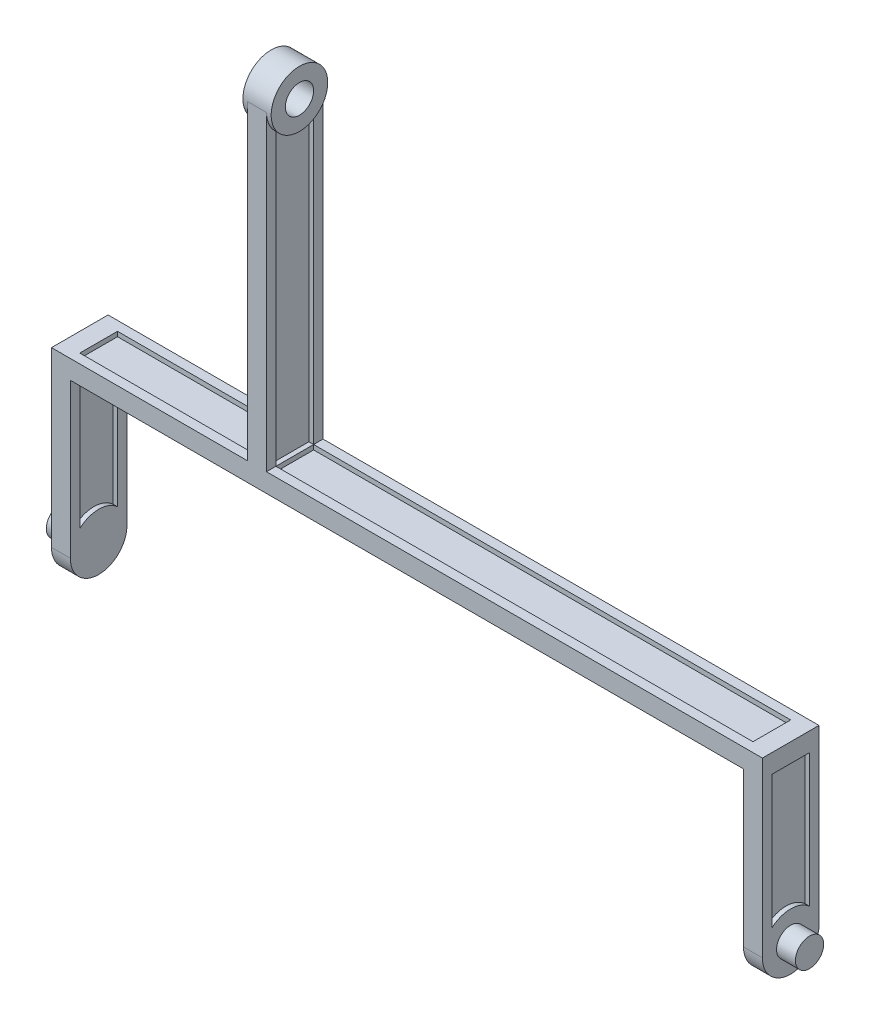
from build123d import *

# Parameters (mm, degrees)
SKETCH_2_R           = 30
SKETCH_2_R_2         = 15
EXTRUDE_1_DEPTH      = 15
EXTRUDE_2_DEPTH      = 10
CUT_EXTRUDE_1_DEPTH  = 5
CUT_EXTRUDE_START    = -5
CUT_EXTRUDE_2_DEPTH  = 5
EXTRUDE_3_DEPTH      = 536
EXTRUDE_3_DEPTH_BACK = 218
SKETCH_6_W           = 60
SKETCH_6_H           = 20
SKETCH_8_W           = 188
SKETCH_8_H           = 40
SKETCH_8_W_2         = 506
CUT_EXTRUDE_3_DEPTH  = 5
SKETCH_9_W           = 714
SKETCH_9_H           = 40
CUT_EXTRUDE_4_DEPTH  = 5
EXTRUDE_4_DEPTH      = 20
EXTRUDE_START        = -20
EXTRUDE_5_DEPTH      = 20
CUT_EXTRUDE_5_DEPTH  = 5
CUT_EXTRUDE_6_DEPTH  = 5
CUT_EXTRUDE_7_DEPTH  = 5
CUT_EXTRUDE_8_DEPTH  = 5
SKETCH_17_R          = 15
EXTRUDE_6_DEPTH      = 20
SKETCH_18_R          = 15.5
EXTRUDE_7_DEPTH      = 20


with BuildPart() as part:
    # 草图2 → 凸台-拉伸1 (new, symmetric)
    with BuildSketch(Plane(origin=(0, 0, 0), x_dir=(0, 0, -1), z_dir=(1, 0, 0))):
        with Locations((0, 34.284448819)):
            Circle(SKETCH_2_R)
        with Locations((0, 34.284448819)):
            Circle(SKETCH_2_R_2, mode=Mode.SUBTRACT)
    extrude(amount=EXTRUDE_1_DEPTH, both=True)

    # 草图3 → 凸台-拉伸2 (add, symmetric)
    with BuildSketch(Plane(origin=(0, 0, 0), x_dir=(0, 0, -1), z_dir=(1, 0, 0))):
        with BuildLine():
            Line((-30, 34.284448819), (-30, -315.715551181))
            Line((-30, -315.715551181), (30, -315.715551181))
            Line((30, -315.715551181), (30, 34.284448819))
            ThreePointArc((30, 34.284448819), (0, 4.284448819), (-30, 34.284448819))
        make_face()
    extrude(amount=EXTRUDE_2_DEPTH, both=True)

    # 草图4 → 切除-拉伸1 (cut)
    with BuildSketch(Plane(origin=(10, 0, 0), x_dir=(0, 0, -1), z_dir=(1, 0, 0))):
        with BuildLine():
            Line((-20, -315.715551181), (-20, 11.923769044))
            ThreePointArc((-20, 11.923769044), (0, 4.284448819), (20, 11.923769044))
            Line((20, 11.923769044), (20, -315.715551181))
            Line((20, -315.715551181), (-20, -315.715551181))
        make_face()
    extrude(amount=-CUT_EXTRUDE_1_DEPTH, mode=Mode.SUBTRACT)

    # 草图5 → 切除-拉伸2 (cut)
    with BuildSketch(Plane.ZY.offset(10).offset(CUT_EXTRUDE_START)):
        with BuildLine():
            Line((-20, 11.923769044), (-20, -315.715551181))
            Line((-20, -315.715551181), (20, -315.715551181))
            Line((20, -315.715551181), (20, 11.923769044))
            ThreePointArc((20, 11.923769044), (0, 4.284448819), (-20, 11.923769044))
        make_face()
    extrude(amount=CUT_EXTRUDE_2_DEPTH, mode=Mode.SUBTRACT)

    # 草图6 → 凸台-拉伸3 (add, two sides: drawn at the far end of the back side and taken through both)
    with BuildSketch(Plane(origin=(0, 0, 0), x_dir=(0, 0, -1), z_dir=(1, 0, 0)).offset(-EXTRUDE_3_DEPTH_BACK)):
        with Locations((0, -305.715551181)):
            Rectangle(SKETCH_6_W, SKETCH_6_H)
    extrude(amount=EXTRUDE_3_DEPTH + EXTRUDE_3_DEPTH_BACK)

    # 草图8 → 切除-拉伸3 (cut)
    with BuildSketch(Plane(origin=(0, -295.715551181, 0), x_dir=(1, 0, 0), z_dir=(0, 1, 0))):
        with Locations((-104, 0)):
            Rectangle(SKETCH_8_W, SKETCH_8_H)
        with Locations((263, 0)):
            Rectangle(SKETCH_8_W_2, SKETCH_8_H)
    extrude(amount=-CUT_EXTRUDE_3_DEPTH, mode=Mode.SUBTRACT)

    # 草图9 → 切除-拉伸4 (cut)
    with BuildSketch(Plane.XZ.offset(315.715551181)):
        with Locations((159, 0)):
            Rectangle(SKETCH_9_W, SKETCH_9_H)
    extrude(amount=-CUT_EXTRUDE_4_DEPTH, mode=Mode.SUBTRACT)

    # 草图11 → 凸台-拉伸4 (add)
    with BuildSketch(Plane(origin=(536, 0, 0), x_dir=(0, 0, -1), z_dir=(1, 0, 0))):
        with BuildLine():
            Line((30, -479.215551181), (30, -315.715551181))
            Line((30, -315.715551181), (-30, -315.715551181))
            Line((-30, -315.715551181), (-30, -479.215551181))
            ThreePointArc((-30, -479.215551181), (0, -509.215551181), (30, -479.215551181))
        make_face()
    extrude(amount=-EXTRUDE_4_DEPTH)

    # 草图12 → 凸台-拉伸5 (add)
    with BuildSketch(Plane.ZY.offset(218).offset(EXTRUDE_START)):
        with BuildLine():
            Line((-30, -315.715551181), (30, -315.715551181))
            Line((30, -315.715551181), (30, -479.215551181))
            ThreePointArc((30, -479.215551181), (0, -509.215551181), (-30, -479.215551181))
            Line((-30, -479.215551181), (-30, -315.715551181))
        make_face()
    extrude(amount=EXTRUDE_5_DEPTH)

    # 草图13 → 切除-拉伸5 (cut)
    with BuildSketch(Plane.ZY.offset(218).offset(CUT_EXTRUDE_START)):
        with BuildLine():
            Line((-20, -315.715551181), (20, -315.715551181))
            Line((20, -315.715551181), (20, -456.854871406))
            ThreePointArc((20, -456.854871406), (0, -449.215551181), (-20, -456.854871406))
            Line((-20, -456.854871406), (-20, -315.715551181))
        make_face()
    extrude(amount=CUT_EXTRUDE_5_DEPTH, mode=Mode.SUBTRACT)

    # 草图14 → 切除-拉伸6 (cut)
    with BuildSketch(Plane(origin=(-198, 0, 0), x_dir=(0, 0, -1), z_dir=(1, 0, 0))):
        with BuildLine():
            Line((-20, -456.854871406), (-20, -315.715551181))
            Line((-20, -315.715551181), (20, -315.715551181))
            Line((20, -315.715551181), (20, -456.854871406))
            ThreePointArc((20, -456.854871406), (0, -449.215551181), (-20, -456.854871406))
        make_face()
    extrude(amount=-CUT_EXTRUDE_6_DEPTH, mode=Mode.SUBTRACT)

    # 草图15 → 切除-拉伸7 (cut)
    with BuildSketch(Plane(origin=(536, 0, 0), x_dir=(0, 0, -1), z_dir=(1, 0, 0))):
        with BuildLine():
            Line((-20, -456.854871406), (-20, -315.715551181))
            Line((-20, -315.715551181), (20, -315.715551181))
            Line((20, -315.715551181), (20, -456.854871406))
            ThreePointArc((20, -456.854871406), (0, -449.215551181), (-20, -456.854871406))
        make_face()
    extrude(amount=-CUT_EXTRUDE_7_DEPTH, mode=Mode.SUBTRACT)

    # 草图16 → 切除-拉伸8 (cut)
    with BuildSketch(Plane.ZY.offset(-516).offset(CUT_EXTRUDE_START)):
        with BuildLine():
            Line((-20, -456.854871406), (-20, -315.715551181))
            Line((-20, -315.715551181), (20, -315.715551181))
            Line((20, -315.715551181), (20, -456.854871406))
            ThreePointArc((20, -456.854871406), (0, -449.215551181), (-20, -456.854871406))
        make_face()
    extrude(amount=CUT_EXTRUDE_8_DEPTH, mode=Mode.SUBTRACT)

    # 草图17 → 凸台-拉伸6 (add)
    with BuildSketch(Plane(origin=(536, 0, 0), x_dir=(0, 0, -1), z_dir=(1, 0, 0))):
        with Locations(Location((0, -479.215551181, 0), (0, 0, 180))):
            Circle(SKETCH_17_R)
    extrude(amount=EXTRUDE_6_DEPTH)

    # 草图18 → 凸台-拉伸7 (add)
    with BuildSketch(Plane.ZY.offset(218)):
        with Locations((0, -479.215551181)):
            Circle(SKETCH_18_R)
    extrude(amount=EXTRUDE_7_DEPTH)


solid = part.part
